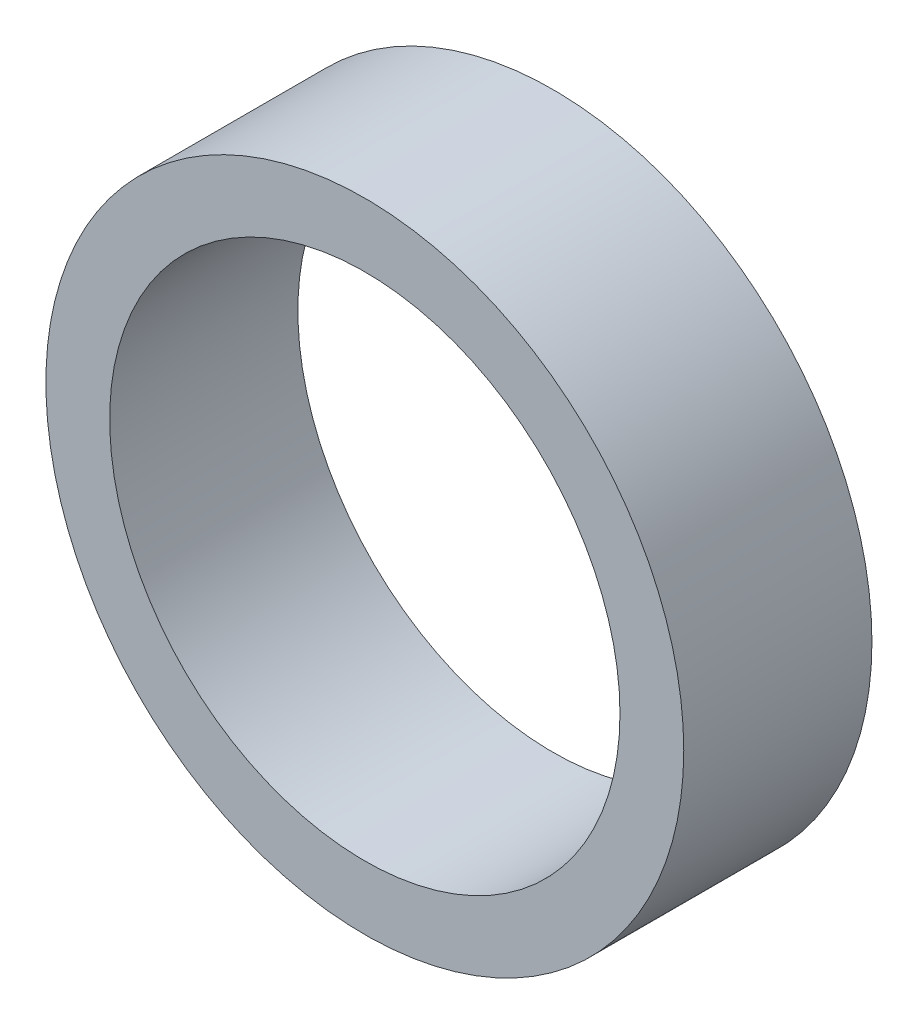
SolidWorks part; units mm, degrees
ref_plane "Front Plane" through (0, 0, 0) normal (0, 0, 1) x (1, 0, 0)
ref_plane "Top Plane" through (0, 0, 0) normal (0, 1, 0) x (1, 0, 0)
ref_plane "Right Plane" through (0, 0, 0) normal (1, 0, 0) x (0, 0, -1)
sketch "Sketch1" plane through (0, 0, 0) normal (0, 0, 1) x (1, 0, 0)
  circle A0 centre (0, 0) radius 40
  circle A1 centre (0, 0) radius 50
  dimension "D1" = 80
  dimension "D2" = 100
extrude "Boss-Extrude1" add sketch "Sketch1" along normal blind 29.5
